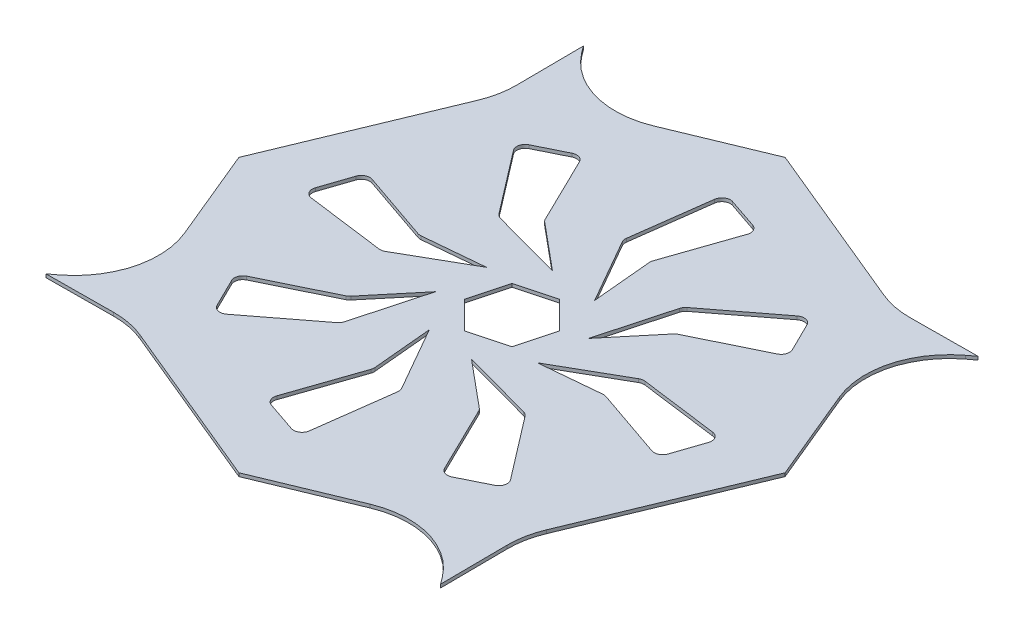
from build123d import *

# Parameters (mm, degrees)
BOSS_EXTRUDE1_DEPTH = 2
CUT_EXTRUDE1_DEPTH  = 10
CUT_EXTRUDE2_DEPTH  = 10
BOSS_EXTRUDE2_DEPTH = 2
FILLET1_R           = 50


with BuildPart() as part:
    # Sketch1 → Boss-Extrude1 (new body)
    with BuildSketch(Plane(origin=(0, 0, 0), x_dir=(1, 0, 0), z_dir=(0, 1, 0))):
        Polygon((114.80502971, -114.80502971), (162.358830044, 0), (114.80502971, 114.80502971), (0, 162.358830044), (-114.80502971, 114.80502971), (-162.358830044, 0), (-114.80502971, -114.80502971), (0, -162.358830044), align=None)
    extrude(amount=BOSS_EXTRUDE1_DEPTH)

    # Sketch2 → Cut-Extrude1 (cut)
    with BuildSketch(Plane(origin=(0, 2, 0), x_dir=(1, 0, 0), z_dir=(0, 1, 0))):
        Polygon((22.307101433, 5.977169814), (5.977169814, 22.307101433), (-16.329931619, 16.329931619), (-22.307101433, -5.977169814), (-5.977169814, -22.307101433), (16.329931619, -16.329931619), align=None)
    extrude(amount=-CUT_EXTRUDE1_DEPTH, mode=Mode.SUBTRACT)

    # Sketch3 → Cut-Extrude2 (cut)
    with BuildSketch(Plane(origin=(0, 2, 0), x_dir=(1, 0, 0), z_dir=(0, 1, 0))):
        with BuildLine():
            Line((7.180747689, 123.974968015), (25.207285, 117.858821427))
            ThreePointArc((25.207285, 117.858821427), (28.089576698, 115.326406795), (28.328747659, 111.497108353))
            Line((28.328747659, 111.497108353), (13.99872444, 69.850478373))
            ThreePointArc((13.99872444, 69.850478373), (13.762569524, 68.82175425), (13.747623306, 67.766377979))
            Line((13.747623306, 67.766377979), (17.02042887, 32.130840461))
            Line((17.02042887, 32.130840461), (-4.884764675, 70.429589412))
            ThreePointArc((-4.884764675, 70.429589412), (-5.450629901, 71.947522663), (-5.501487679, 73.566700941))
            Line((-5.501487679, 73.566700941), (0.617313414, 119.89476636))
            ThreePointArc((0.617313414, 119.89476636), (2.934488498, 123.486434711), (7.180747689, 123.974968015))
        make_face()
        with BuildLine():
            Line((92.741095966, 82.585985196), (101.163014013, 65.514529695))
            ThreePointArc((101.163014013, 65.514529695), (101.410414459, 61.68575413), (98.871810971, 58.808911827))
            Line((98.871810971, 58.808911827), (59.290339906, 39.493153947))
            ThreePointArc((59.290339906, 39.493153947), (58.395935361, 38.932722886), (57.63910307, 38.197027741))
            Line((57.63910307, 38.197027741), (34.755195848, 10.684674503))
            Line((34.755195848, 10.684674503), (46.347190043, 53.255290495))
            ThreePointArc((46.347190043, 53.255290495), (47.0204038, 54.72875853), (48.129373861, 55.909652349))
            Line((48.129373861, 55.909652349), (85.214908823, 84.34189582))
            ThreePointArc((85.214908823, 84.34189582), (89.393092084, 85.243098653), (92.741095966, 82.585985196))
        make_face()
        with BuildLine():
            Line((123.974968015, -7.180747689), (117.858821427, -25.207285))
            ThreePointArc((117.858821427, -25.207285), (115.326406795, -28.089576698), (111.497108353, -28.328747659))
            Line((111.497108353, -28.328747659), (69.850478373, -13.99872444))
            ThreePointArc((69.850478373, -13.99872444), (68.82175425, -13.762569524), (67.766377979, -13.747623306))
            Line((67.766377979, -13.747623306), (32.130840461, -17.02042887))
            Line((32.130840461, -17.02042887), (70.429589412, 4.884764675))
            ThreePointArc((70.429589412, 4.884764675), (71.947522663, 5.450629901), (73.566700941, 5.501487679))
            Line((73.566700941, 5.501487679), (119.89476636, -0.617313414))
            ThreePointArc((119.89476636, -0.617313414), (123.486434711, -2.934488498), (123.974968015, -7.180747689))
        make_face()
        with BuildLine():
            Line((82.585985196, -92.741095966), (65.514529695, -101.163014013))
            ThreePointArc((65.514529695, -101.163014013), (61.68575413, -101.410414459), (58.808911827, -98.871810971))
            Line((58.808911827, -98.871810971), (39.493153947, -59.290339906))
            ThreePointArc((39.493153947, -59.290339906), (38.932722886, -58.395935361), (38.197027741, -57.63910307))
            Line((38.197027741, -57.63910307), (10.684674503, -34.755195848))
            Line((10.684674503, -34.755195848), (53.255290495, -46.347190043))
            ThreePointArc((53.255290495, -46.347190043), (54.72875853, -47.0204038), (55.909652349, -48.129373861))
            Line((55.909652349, -48.129373861), (84.34189582, -85.214908823))
            ThreePointArc((84.34189582, -85.214908823), (85.243098653, -89.393092084), (82.585985196, -92.741095966))
        make_face()
        with BuildLine():
            Line((-7.180747689, -123.974968015), (-25.207285, -117.858821427))
            ThreePointArc((-25.207285, -117.858821427), (-28.089576698, -115.326406795), (-28.328747659, -111.497108353))
            Line((-28.328747659, -111.497108353), (-13.99872444, -69.850478373))
            ThreePointArc((-13.99872444, -69.850478373), (-13.762569524, -68.82175425), (-13.747623306, -67.766377979))
            Line((-13.747623306, -67.766377979), (-17.02042887, -32.130840461))
            Line((-17.02042887, -32.130840461), (4.884764675, -70.429589412))
            ThreePointArc((4.884764675, -70.429589412), (5.450629901, -71.947522663), (5.501487679, -73.566700941))
            Line((5.501487679, -73.566700941), (-0.617313414, -119.89476636))
            ThreePointArc((-0.617313414, -119.89476636), (-2.934488497, -123.486434711), (-7.180747689, -123.974968015))
        make_face()
        with BuildLine():
            Line((-92.741095966, -82.585985196), (-101.163014013, -65.514529695))
            ThreePointArc((-101.163014013, -65.514529695), (-101.410414459, -61.68575413), (-98.871810971, -58.808911827))
            Line((-98.871810971, -58.808911827), (-59.290339906, -39.493153947))
            ThreePointArc((-59.290339906, -39.493153947), (-58.395935361, -38.932722886), (-57.63910307, -38.197027741))
            Line((-57.63910307, -38.197027741), (-34.755195848, -10.684674503))
            Line((-34.755195848, -10.684674503), (-46.347190043, -53.255290495))
            ThreePointArc((-46.347190043, -53.255290495), (-47.0204038, -54.72875853), (-48.129373861, -55.909652349))
            Line((-48.129373861, -55.909652349), (-85.214908823, -84.34189582))
            ThreePointArc((-85.214908823, -84.34189582), (-89.393092084, -85.243098653), (-92.741095966, -82.585985196))
        make_face()
        with BuildLine():
            Line((-123.974968015, 7.180747689), (-117.858821427, 25.207285))
            ThreePointArc((-117.858821427, 25.207285), (-115.326406795, 28.089576698), (-111.497108353, 28.328747659))
            Line((-111.497108353, 28.328747659), (-69.850478373, 13.99872444))
            ThreePointArc((-69.850478373, 13.99872444), (-68.82175425, 13.762569524), (-67.766377979, 13.747623306))
            Line((-67.766377979, 13.747623306), (-32.130840461, 17.02042887))
            Line((-32.130840461, 17.02042887), (-70.429589412, -4.884764675))
            ThreePointArc((-70.429589412, -4.884764675), (-71.947522663, -5.450629901), (-73.566700941, -5.501487679))
            Line((-73.566700941, -5.501487679), (-119.89476636, 0.617313414))
            ThreePointArc((-119.89476636, 0.617313414), (-123.486434711, 2.934488497), (-123.974968015, 7.180747689))
        make_face()
        with BuildLine():
            Line((-82.585985196, 92.741095966), (-65.514529695, 101.163014013))
            ThreePointArc((-65.514529695, 101.163014013), (-61.68575413, 101.410414459), (-58.808911827, 98.871810971))
            Line((-58.808911827, 98.871810971), (-39.493153947, 59.290339906))
            ThreePointArc((-39.493153947, 59.290339906), (-38.932722886, 58.395935361), (-38.197027741, 57.63910307))
            Line((-38.197027741, 57.63910307), (-10.684674503, 34.755195848))
            Line((-10.684674503, 34.755195848), (-53.255290495, 46.347190043))
            ThreePointArc((-53.255290495, 46.347190043), (-54.72875853, 47.0204038), (-55.909652349, 48.129373861))
            Line((-55.909652349, 48.129373861), (-84.34189582, 85.214908823))
            ThreePointArc((-84.34189582, 85.214908823), (-85.243098653, 89.393092084), (-82.585985196, 92.741095966))
        make_face()
    extrude(amount=-CUT_EXTRUDE2_DEPTH, mode=Mode.SUBTRACT)

    # Sketch6 → Boss-Extrude2 (add)
    with BuildSketch(Plane(origin=(0, 2, 0), x_dir=(1, 0, 0), z_dir=(0, 1, 0))):
        Polygon((-116.910273848, 109.722520758), (-117.296113887, 159.722520758), (-90.835857438, 124.733385943), (-114.80502971, 114.80502971), align=None)
        Polygon((109.722520758, 116.910273848), (159.722520758, 117.296113887), (124.733385943, 90.835857438), (114.80502971, 114.80502971), align=None)
        Polygon((116.910273848, -109.722520758), (117.296113887, -159.722520758), (90.835857438, -124.733385943), (114.80502971, -114.80502971), align=None)
        Polygon((-109.722520758, -116.910273848), (-159.722520758, -117.296113887), (-124.733385943, -90.835857438), (-114.80502971, -114.80502971), align=None)
    extrude(amount=-BOSS_EXTRUDE2_DEPTH)

    # Fillet1
    fillet1_edges = [part.edges().sort_by_distance(p)[0] for p in [
        (-116.910273848, 1, -109.722520758),
        (-90.835857438, 1, -124.733385943),
        (109.722520758, 1, -116.910273848),
        (124.733385943, 1, -90.835857438),
        (116.910273848, 1, 109.722520758),
        (90.835857438, 1, 124.733385943),
        (-109.722520758, 1, 116.910273848),
        (-124.733385943, 1, 90.835857438),
    ]]
    fillet(fillet1_edges, radius=FILLET1_R)


solid = part.part
